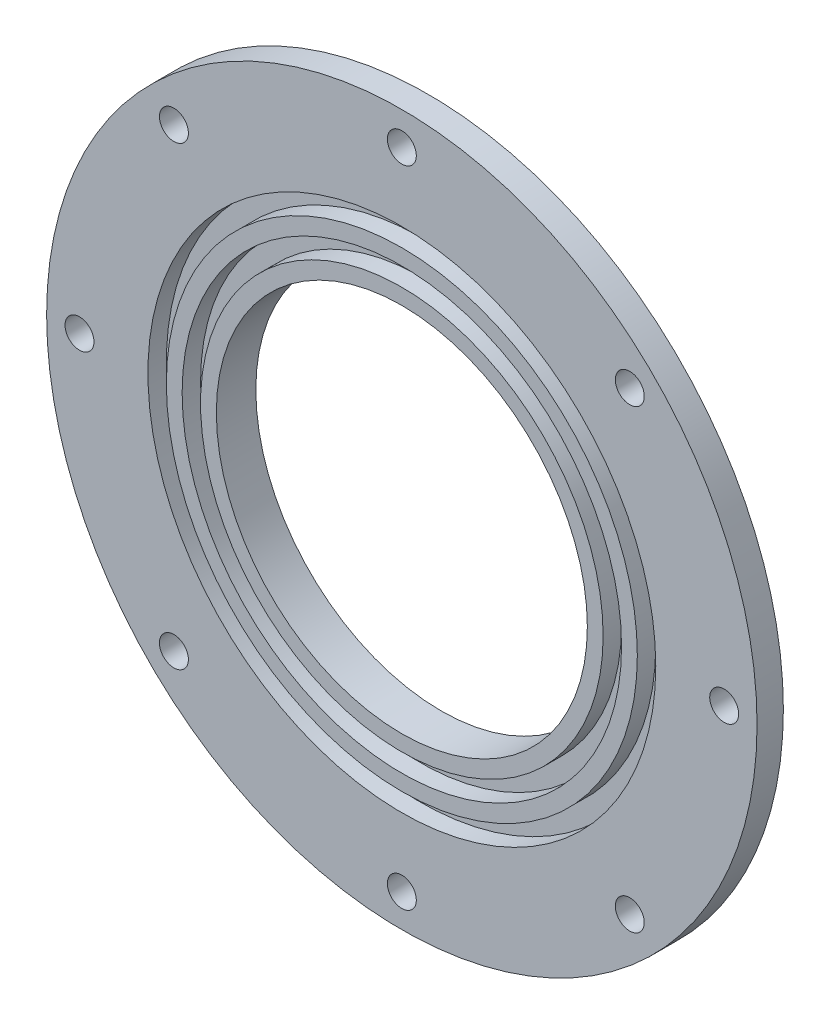
SolidWorks part; units mm, degrees
material "灰铸铁 HT150 "
ref_plane "Front Plane" through (0, 0, 0) normal (0, 0, 1) x (1, 0, 0)
ref_plane "Top Plane" through (0, 0, 0) normal (0, 1, 0) x (1, 0, 0)
ref_plane "Right Plane" through (0, 0, 0) normal (1, 0, 0) x (0, 0, -1)
sketch "Sketch1" plane through (0, 0, 0) normal (1, 0, 0) x (0, 0, -1)
  line L0 (0, 0) -> (242.296, 0) construction
  line L1 (0, 141) -> (0, 153)
  line L2 (0, 270) -> (20, 270)
  line L3 (20, 270) -> (20, 220)
  line L4 (20, 220) -> (45, 220)
  line L5 (45, 220) -> (45, 200)
  line L6 (45, 200) -> (30, 200)
  line L7 (30, 200) -> (30, 141)
  line L8 (30, 141) -> (0, 141)
  line L13 (0, 167) -> (0, 179)
  line L14 (0, 167) -> (14, 167)
  line L15 (0, 153) -> (14, 153)
  line L16 (14, 167) -> (14, 153)
  line L17 (0, 193) -> (0, 270)
  line L18 (0, 193) -> (14, 193)
  line L19 (0, 179) -> (14, 179)
  line L20 (14, 193) -> (14, 179)
  dimension "D1" = 141
  dimension "D2" = 153
  dimension "D3" = 167
  dimension "D4" = 179
  dimension "D5" = 193
  dimension "D6" = 270
  dimension "D7" = 200
  dimension "D8" = 220
  dimension "D9" = 45
  dimension "D10" = 25
  dimension "D11" = 14
  dimension "D12" = 30
revolve "Revolve1" add sketch "Sketch1" angle 360 about L0
sketch "Sketch2" plane through (0, 0, 0) normal (0, 0, 1) x (1, 0, 0)
  line L0 (0, 0) -> (0, 245) construction
  circle A0 centre (0, 245) radius 11
  dimension "D2" = 22
  dimension "D1" = 245
extrude "Cut-Extrude1" cut sketch "Sketch2" against normal blind 41
pattern_circular "CirPattern1" count 8 over 360 about axis through (0, 0, 0) along (0, 0, 1) of "Cut-Extrude1"
